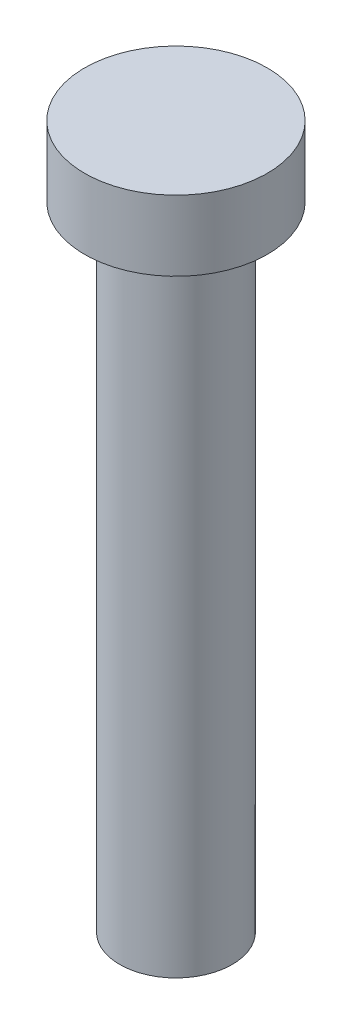
SolidWorks part; units mm, degrees
ref_plane "Front Plane" through (0, 0, 0) normal (0, 0, 1) x (1, 0, 0)
ref_plane "Top Plane" through (0, 0, 0) normal (0, 1, 0) x (1, 0, 0)
ref_plane "Right Plane" through (0, 0, 0) normal (1, 0, 0) x (0, 0, -1)
sketch "Sketch1" plane through (0, 0, 0) normal (0, 0, 1) x (1, 0, 0)
  line L0 (0, 0) -> (0, 50)
  line L1 (0, 50) -> (6.5, 50)
  line L2 (6.5, 50) -> (6.5, 45)
  line L3 (6.5, 45) -> (4, 45)
  line L4 (4, 45) -> (4, 0)
  line L5 (4, 0) -> (0, 0)
  dimension "D1" = 45
  dimension "D2" = 4
  dimension "D3" = 6.5
  dimension "D4" = 5
revolve "Revolve1" add sketch "Sketch1" angle 360 about L0
